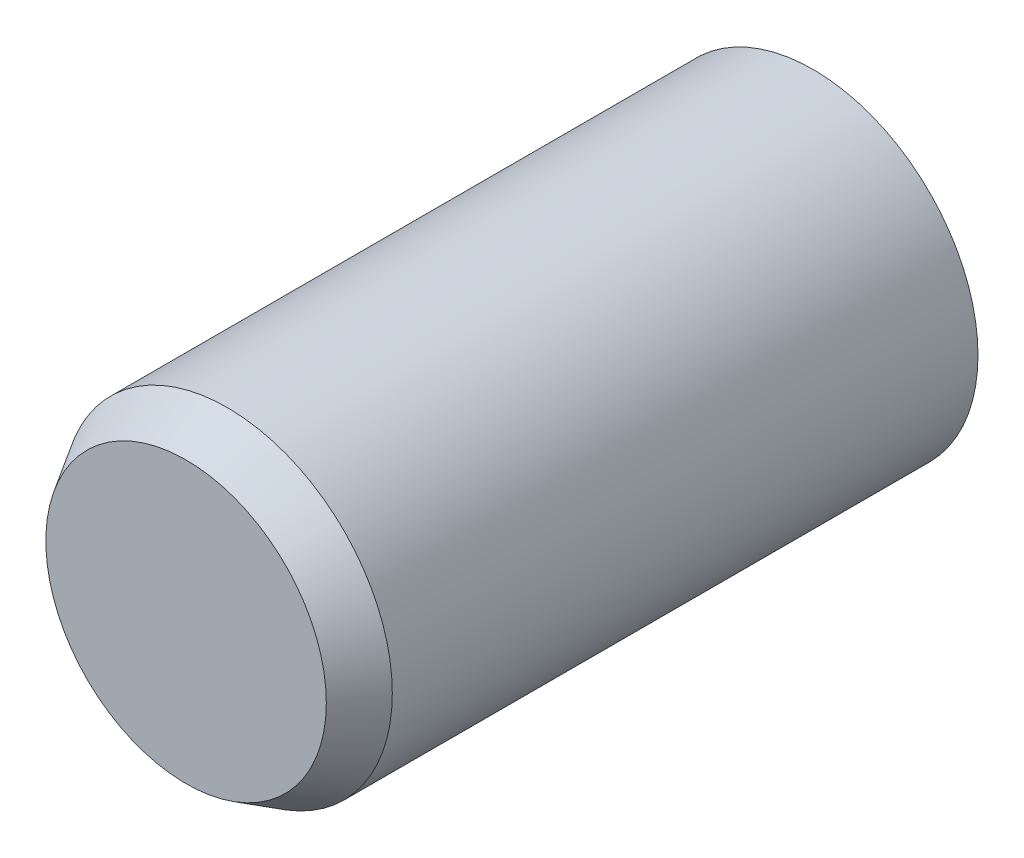
SolidWorks part; units mm, degrees
material "S45C"
ref_plane "Front Plane" through (0, 0, 0) normal (0, 0, 1) x (1, 0, 0)
ref_plane "Top Plane" through (0, 0, 0) normal (0, 1, 0) x (1, 0, 0)
ref_plane "Right Plane" through (0, 0, 0) normal (1, 0, 0) x (0, 0, -1)
sketch "Sketch1" plane through (0, 0, 0) normal (0, 0, 1) x (1, 0, 0)
  circle A0 centre (0, 0) radius 40
  dimension "D1" = 80
extrude "Boss-Extrude1" add sketch "Sketch1" along normal blind 152
chamfer "Chamfer1" distance 10 distance2 6 1 edges at (40, 0, 152)
hole_wizard "M6 Tapped Hole1" positions "Sketch4" profile "Sketch3" tap size "M6" standard "GB"
sketch "Sketch4" plane through (0, 0, 0) normal (0, 0, -1) x (-1, 0, 0)
  point P0 (0, 0)
sketch "Sketch3" plane through (0, 0, 0) normal (1, 0, 0) x (0, 1, 0)
  line L0 (0, 0) -> (0, 18.5022)
  line L1 (0, 18.5022) -> (2.5, 17)
  line L2 (2.5, 17) -> (2.5, 0)
  line L5 (2.5, 0) -> (0, 0)
  line L10 (0, 18.5022) -> (-2.5, 17) construction
  line L11 (0, -6.35) -> (0, 107.95) construction
  dimension "螺纹孔钻头直径" = 5
  dimension "螺纹孔钻头深度" = 17
  dimension "导头角度" = 118
cosmetic thread "Hole thread1"
